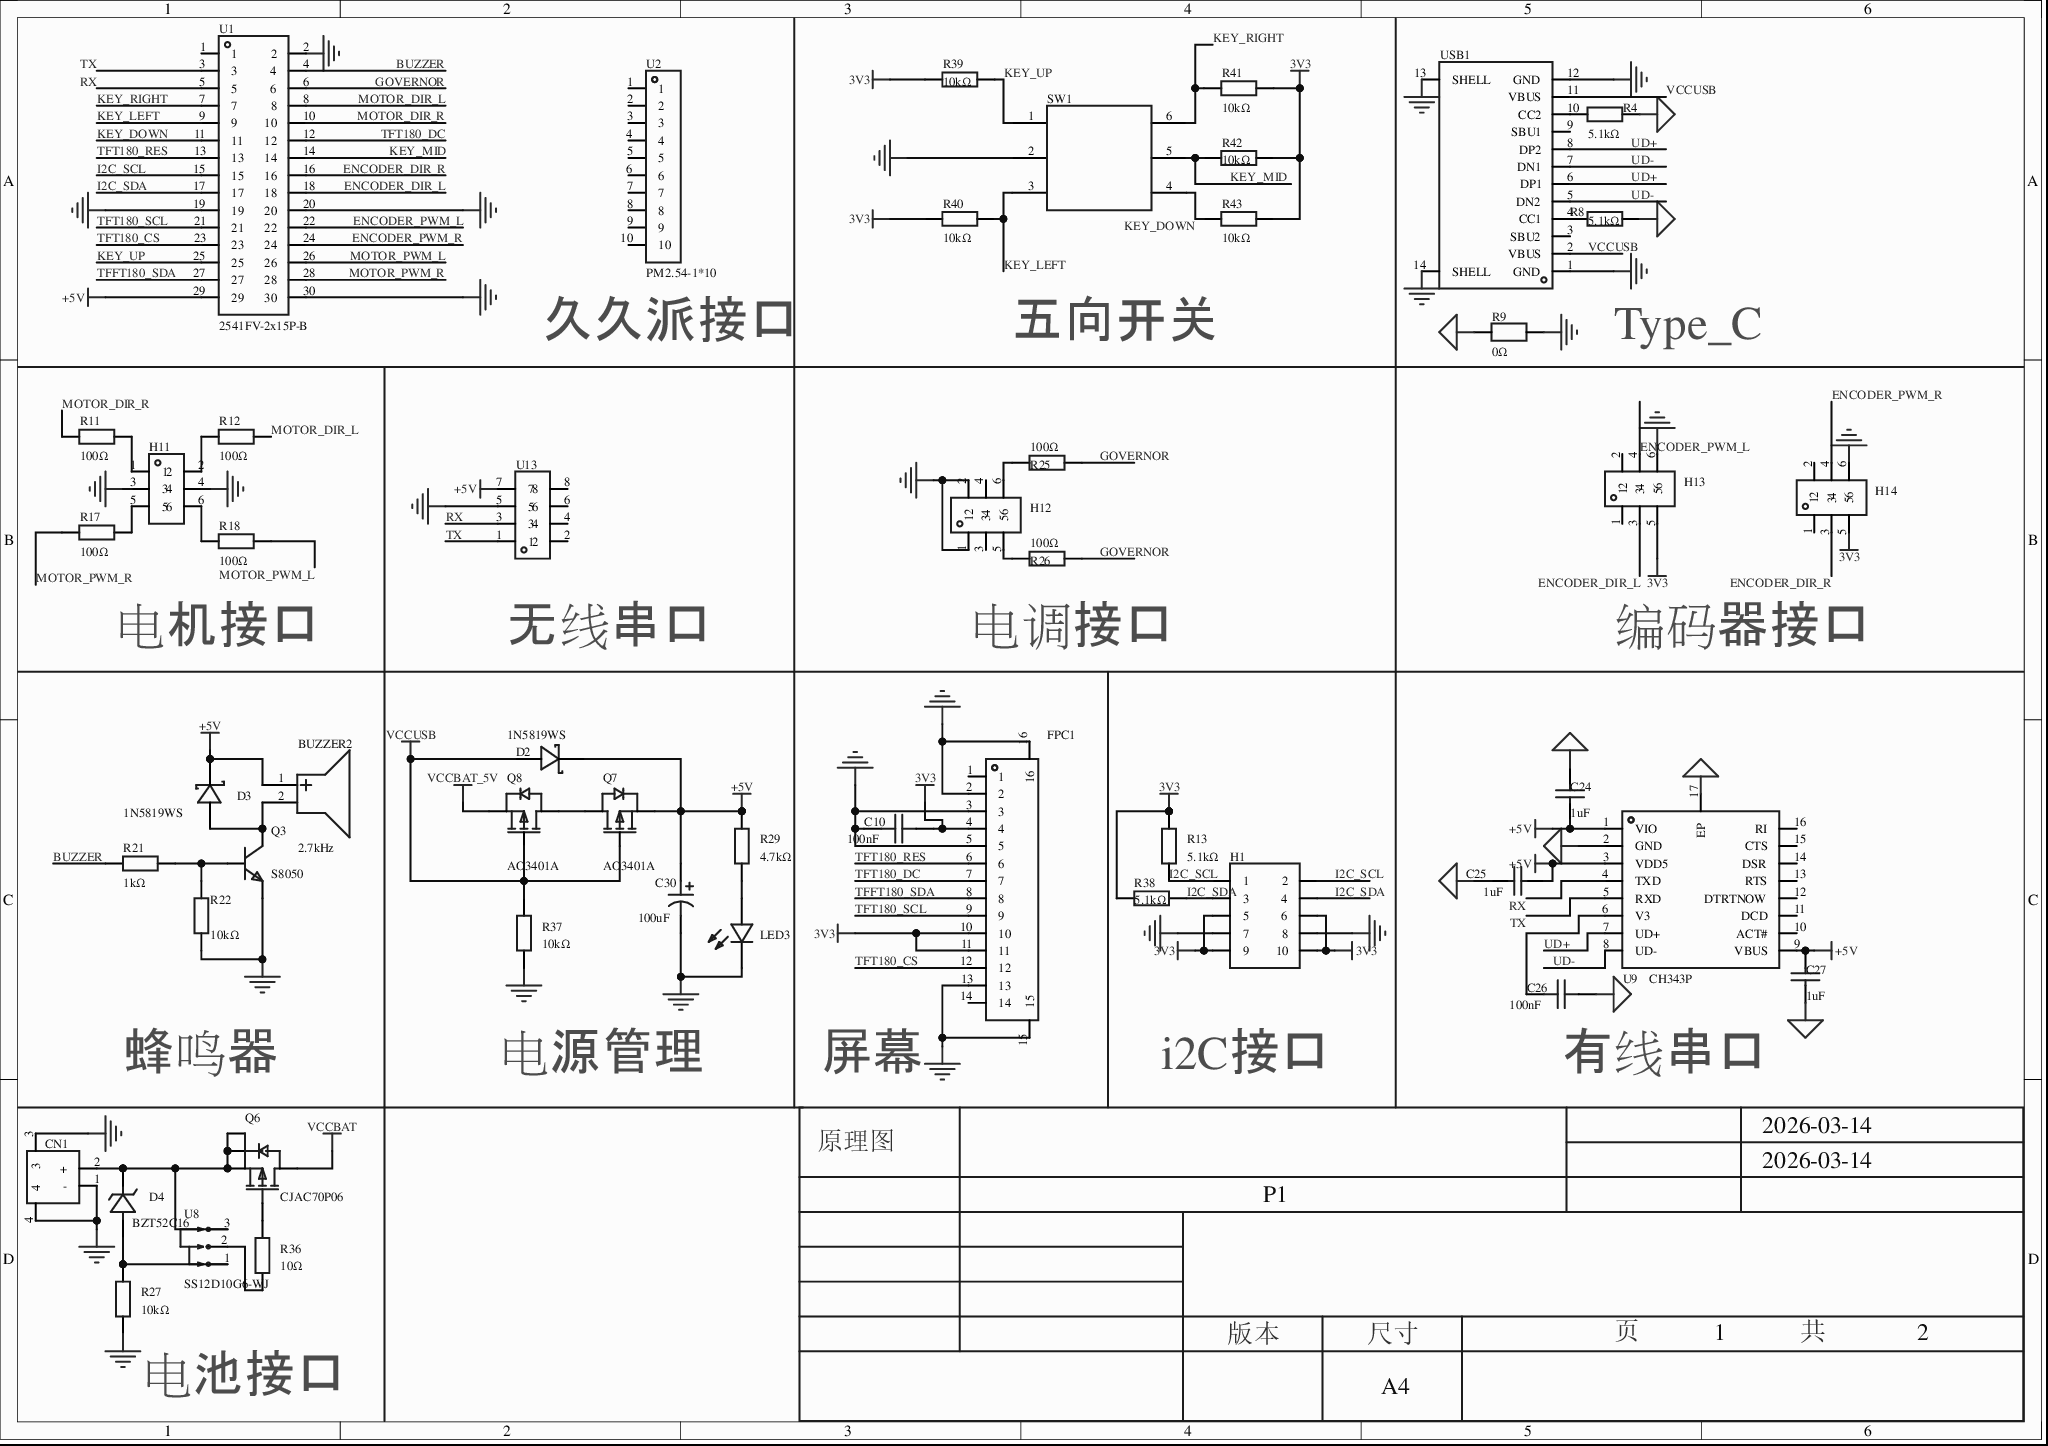
[diagram p0: MISC51977-3.schdoc]
# Altium project MISC51977-2.PrjPcb (part 1 of 2)
2 sheets, 74 parts. Net scope: global (net labels, ports and power ports of the same name join across sheets).
Board file: MISC51977.pcbdoc
Sheets:
  MISC51977-3.schdoc
  MISC51977-4.schdoc

## Sheet MISC51977-3.schdoc
size 297 x 209 mm; Version: V1.0; @Project Name: MISC51977; @Page Count: 2; @Update Date: 2026-03-14; @Create Date: 2026-03-14; @Schematic Name: MISC51977; @Page No: 1; @Board Name: MISC51977; @Create Time: 15:58:27; @Update Time: 22:07:32

### Parts
BUZZER2  2.7kHz  [BUZ-SMD_GSC9032RB]
C10  100nF  [C0603]
C24  1uF  [C0805]
C25  1uF  [C0805]
C26  100nF  [C0603]
C27  1uF  [C0805]
C30  100uF  [CAP-SMD_BD6.3-L6.6-W6.6-FD-1]
CN1  XT30PW-M30.G.Y  [CONN-TH_XT30PW-M]  (value not drawn)
D2  1N5819WS  [SOD-323_L1.8-W1.3-LS2.5-RD]
D3  1N5819WS  [SOD-323_L1.8-W1.3-LS2.5-RD]
D4  BZT52C16  [SOD-123_L2.7-W1.6-LS3.7-RD]
FPC1  HC-FPC-05-09-14RLTAG  [FPC-SMD_14P-P0.50_HC-FPC-05-09-14RLTAG]  (value not drawn)
H1  (no value)  [HDR-TH_10P-P2.54-V-F-R2-C5-S2.54]
H11  HX PZ2.54-2x3P TP  [HDR-SMD_6P-P2.54-V-M-R2-C3-LS7.2_M20-8760342]  (value not drawn)
H12  HX PZ2.54-2x3P TP  [HDR-SMD_6P-P2.54-V-M-R2-C3-LS7.2_M20-8760342]  (value not drawn)
H13  PZ254V-12-6P  [HDR-TH_6P-P2.54-V-M-R2-C3-S2.54]  (value not drawn)
H14  PZ254V-12-6P  [HDR-TH_6P-P2.54-V-M-R2-C3-S2.54]  (value not drawn)
LED3  NCD0603R1  [LED0603-RD_RED]  (value not drawn)
Q3  S8050  [SOT-23-3_L2.9-W1.6-P1.90-LS2.8-BR]
Q6  CJAC70P06  [TDSON-8_L5.9-W5.2-P1.27-BL]
Q7  AO3401A  [SOT-23_L2.9-W1.3-P1.90-LS2.4-BR]
Q8  AO3401A  [SOT-23_L2.9-W1.3-P1.90-LS2.4-BR]
R4  5.1kΩ  [R0603]
R8  5.1kΩ  [R0603]
R9  0Ω  [R1206]
R11  100Ω  [R0603]
R12  100Ω  [R0603]
R13  5.1kΩ  [R0603]
R17  100Ω  [R0603]
R18  100Ω  [R0603]
R21  1kΩ  [R0603]
R22  10kΩ  [R0603]
R25  100Ω  [R0603]
R26  100Ω  [R0603]
R27  10kΩ  [R0603]
R29  4.7kΩ  [R0603]
R36  10Ω  [R0603]
R37  10kΩ  [R0603]
R38  5.1kΩ  [R0603]
R39  10kΩ  [R0603]
R40  10kΩ  [R0603]
R41  10kΩ  [R0603]
R42  10kΩ  [R0603]
R43  10kΩ  [R0603]
SW1  7*7*5-6P-L WX  [SW-SMD_8P-L7.0-W7.0-P1.40-LS7.4-TL]  (value not drawn)
U1  2541FV-2x15P-B  [HDR-TH_30P-P2.54-V-F-R2-C15-S2.54]
U2  PM2.54-1*10  [HDR-TH_10P-P2.54-V-F]
U8  SS12D10G6-WJ  [SW-TH_3P-P4.80_HX-SS12D10G6-WJ]
U9  CH343P  [TQFN-16_L3.0-W3.0-P0.50-BL-EP1.7]
U13  5BME8-08872-204-W0  [CONN-SMD_5BME8-08872-204-W0]  (value not drawn)
USB1  TYPE-C 16PIN 2MD(073)  [USB-C-SMD_TYPE-C-6PIN-2MD-073]  (value not drawn)

### Nets
3V3: C10.2 FPC1.4 FPC1.10 FPC1.11 H1.5 H1.6 H1.9 H1.10 H13.5 H14.5 R13.2 R38.2 R39.1 R40.1 R41.2 R42.2 R43.2
+5V: BUZZER2.1(+) C24.1 C25.1 C27.2 C30.1 D2.1(K) D3.1(K) Q7.2(S) R29.2 U1.29 U9.1(VIO) U9.3(VDD5) U9.9(VBUS) U13.7
AGND: C24.2 C25.2 C26.2 C27.1 R4.2 R8.2 R9.1 U9.2(GND) U9.17(EP)
GND: C10.1 C30.2 CN1.1(-) CN1.3 CN1.4 FPC1.2 FPC1.3 FPC1.5 FPC1.13 FPC1.15 FPC1.16 H1.7 H1.8 H11.3 H11.4 H12.1 H12.2 H13.6 H14.6 LED3.1(K) Q3.2 R9.2 R22.2 R27.1 R37.1 SW1.2 U1.2 U1.19 U1.20 U1.30 U13.5 USB1.1(GND) USB1.12(GND) USB1.13(SHELL) USB1.14(SHELL)
VCCBAT: Q6.5(D)
VCCBAT_5V: Q8.2(S)
VCCUSB: D2.2(A) Q7.1(G) Q8.1(G) R37.2 USB1.2(VBUS) USB1.11(VBUS)
BUZZER: R21.1 U1.4
ENCODER_DIR_L: H13.3 U1.18
ENCODER_DIR_R: H14.3 U1.16
ENCODER_PWM_L: H13.4 U1.22
ENCODER_PWM_R: H14.4 U1.24
GOVERNOR: R25.2 R26.2 U1.6
I2C_SCL: H1.1 H1.2 R13.1 U1.15
I2C_SDA: H1.3 H1.4 R38.1 U1.17
KEY_DOWN: R43.1 SW1.4 U1.11
KEY_LEFT: R40.2 SW1.3 U1.9
KEY_MID: R42.1 SW1.5 U1.14
KEY_RIGHT: R41.1 SW1.6 U1.7
KEY_UP: R39.2 SW1.1 U1.25
MOTOR_DIR_L: R12.2 U1.8
MOTOR_DIR_R: R11.1 U1.10
MOTOR_PWM_L: R18.2 U1.26
MOTOR_PWM_R: R17.1 U1.28
RX: U1.5 U9.4(TXD) U13.3
TFFT180_SDA: FPC1.8 U1.27
TFT180_CS: FPC1.12 U1.23
TFT180_DC: FPC1.7 U1.12
TFT180_RES: FPC1.6 U1.13
TFT180_SCL: FPC1.9 U1.21
TX: U1.3 U9.5(RXD) U13.1
UD+: U9.7(UD+) USB1.6(DP1) USB1.8(DP2)
UD-: U9.8(UD-) USB1.5(DN2) USB1.7(DN1)
NetBUZZER2_2: BUZZER2.2(-) D3.2(A) Q3.3
NetC26_1: C26.1 U9.6(V3)
NetCN1_2: CN1.2(+) D4.1(K) Q6.1(S) Q6.2(S) Q6.3(S) U8.3
NetD4_2: D4.2(A) R27.2 U8.1
NetH11_1: H11.1 R11.2
NetH11_2: H11.2 R12.1
NetH11_5: H11.5 R17.2
NetH11_6: H11.6 R18.1
NetH12_5: H12.5 R26.1
NetH12_6: H12.6 R25.1
NetLED3_2: LED3.2(A) R29.1
NetQ3_1: Q3.1 R21.2 R22.1
NetQ6_4: Q6.4(G) R36.2
NetQ7_3: Q7.3(D) Q8.3(D)
NetR4_1: R4.1 USB1.10(CC2)
NetR8_1: R8.1 USB1.4(CC1)
NetR36_1: R36.1 U8.2

Not connected (* = marked no-connect by the designer): FPC1 1* 14*; H12 3* 4*; H13 1* 2*; H14 1* 2*; U1 1*; U2 1* 2* 3* 4* 5* 6* 7* 8* 9* 10*; U9 10(ACT#)* 11(DCD)* 12(DTRTNOW)* 13(RTS)* 14(DSR)* 15(CTS)* 16(RI)*; U13 2* 4* 6* 8*; USB1 3(SBU2)* 9(SBU1)*

### Notes on the sheet
- (near U2) 久久派接口
- 五向开关
- Type_C
- 电机接口
- (near U13) 无线串口
- 电调接口
- 编码器接口
- 蜂鸣器
- 电源管理
- 屏幕
- i2C接口
- (near C26) 有线串口
- (near R27) 电池接口
- 2026-03-14
- 原理图
- P1
- 版本
- 尺寸
- A4
- 页
- 1
- 共
- 2

### Library data of the parts
BUZZER2 = GSC9032RB-16R2700: 驱动方式:无源(外部驱动);构造类型:电磁式;额定电压:3.6V;频率:2.7kHz;声压(SPL):85dB;; Manufacturer: INGHAi(赢海); AddInBom: yes; ModelId: 6d10ac767011472d9e367b81df9b4b54; ModelName: BUZ-SMD_BD9.0-H3.2-LS10.5; ModelTransform: 413.385,413.385,0,180,0,0,0.002,-29.532,0; Voltage Rating: 3.6V; Voltage - Supply: 2V~4V; Current Consumption: 80mA; Sound Pressure Level(SPL): 85dB; Symbol: GSC9032RB-16R2700; Device: GSC9032RB-16R2700; LCSC Part Name: 贴片式电磁无源蜂鸣器（外部驱动）; SupplierPart: C255321; ManufacturerPart: GSC9032RB-16R2700; Supplier Footprint: -; JLCPCB Part Class: 扩展库; Datasheet: https://item.szlcsc.com/datasheet/GSC9032RB-16R2700/249273.html; Supplier: LCSC; ConvertToPcb: yes; FootprintName: BUZ-SMD_GSC9032RB; Driver Circuitry: 无源(外部驱动); Technology: 电磁式; Value: 2.7kHz; Diameter(φD): 9mm; Height: 3.5mm; Operating Temperature: -20℃~+80℃; Mounting Type: 贴片
C10 C26 = CGA0603X7R104K500JT: 容值:100nF;精度:±10%;额定电压:50V;材质(温度系数):X7R;; Manufacturer: HRE(芯声); AddInBom: yes; ModelId: ac125912035d415993ca9572d50418b1; ModelName: C0603_L1.6-W0.8-H0.8; ModelTransform: 62.992,31.496,0,0,0,0,0,0,0; Tolerance: ±10%; Voltage Rated: 50V; Temperature Coefficient: X7R; Symbol: CGA0603X7R104K500JT; Device: CGA0603X7R104K500JT; LCSC Part Name: 100nF ±10% 50V; SupplierPart: C6119867; ManufacturerPart: CGA0603X7R104K500JT; Supplier Footprint: 0603; JLCPCB Part Class: 扩展库; Supplier: LCSC; ConvertToPcb: yes; FootprintName: C0603; Value: 100nF
C24 C25 C27 = CL21B105KBFNNNE: 容值:1uF;精度:±10%;额定电压:50V;温度系数:X7R;; Manufacturer: SAMSUNG(三星); AddInBom: yes; ModelId: 1ba041120af144c991958decab20d241; ModelName: C0805_L2.0-W1.3-H1.3; ModelTransform: 78.74,51.181,0,0,0,0,0,0.0005,0; Tolerance: ±10%; Voltage Rating: 50V; Temperature Coefficient: X7R; Symbol: CL21B105KBFNNNE; Device: CL21B105KBFNNNE; LCSC Part Name: 1uF ±10% 50V; SupplierPart: C28323; ManufacturerPart: CL21B105KBFNNNE; Supplier Footprint: 0805; JLCPCB Part Class: 基础库; Datasheet: https://item.szlcsc.com/datasheet/CL21B105KBFNNNE/29074.html; Supplier: LCSC; ConvertToPcb: yes; FootprintName: C0805; Value: 1uF
C30 = JVJ25V100M6x5: 容值:100uF;精度:±20%;额定电压:25V;纹波电流:72mA@120Hz;; Manufacturer: JIERR(捷而瑞); AddInBom: yes; ModelId: 041333f082e2432d92aae8a67d233574; ModelTransform: 299.212,259.842,0,0,0,0,0,0,0; Tolerance: ±20%; Voltage Rating: 25V; Lifetime: 2000hrs@105℃; Symbol: JVJ25V100M6X5; Device: JVJ25V100M6x5; LCSC Part Name: 100uF ±20% 25V; SupplierPart: C46550402; ManufacturerPart: JVJ25V100M6x5; Supplier Footprint: SMD,D6.3xL5.4mm; JLCPCB Part Class: 扩展库; Datasheet: https://item.szlcsc.com/datasheet/JVJ25V100M6x5/48680096.html; Supplier: LCSC; ConvertToPcb: yes; FootprintName: CAP-SMD_BD6.3-L6.6-W6.6-FD-1; ModelName: CAP-SMD_BD6.3-L6.6-W6.6-FD-1; Value: 100uF; Ripple Current: 72mA@120Hz; Diameter: 6.3mm; Height - Seated (Max): 5.4mm; Operating Temperature: -55℃~+105℃
CN1 = XT30PW-M30.G.Y: 类别:-;类型1:-;; Manufacturer: AMASS(艾迈斯); AddInBom: yes; ModelId: 722652c2597f41cd937322584dc4b29b; ModelTransform: 523.621,549.2115,0,0,0,0,-0.005,-39.568,-78.74; RatedVoltage: DC 500V; InterfaceType: 公头; RatedCurrent: 15A; RecommendedWireGauge: 16/18/20AWG; contact resistance: 1.2mΩ; specifications: 2pin; Symbol: XT30PW-M; Device: XT30PW-M30.G.Y; LCSC Part Name: AMASS(艾迈斯)航模插头 卧式弯脚 XT30PW-M公头; SupplierPart: C431092; ManufacturerPart: XT30PW-M30.G.Y; Supplier Footprint: -; JLCPCB Part Class: 扩展库; Datasheet: https://atta.szlcsc.com/upload/public/pdf/source/20220222/6A9F22F7850E25B33E1BE430ADF8560B.pdf; Supplier: LCSC; ConvertToPcb: yes; FootprintName: CONN-TH_XT30PW-M; ModelName: CONN-TH_XT30PW-M; Power: -; Output: -; Input: -; Size: -; Interface: -; Type: 航模插头; Colour: -; MaximumCurrent: -; Type1: -; NumberOfUSBHoles: -; MetalMaterial: -; InsulationMaterial: -; FlameRetardantGrade: -; Belt length: -
D2 D3 = 1N5819WS_C191023: 正向压降(Vf):600mV@1A;直流反向耐压(Vr):40V;整流电流:1A;; Manufacturer: Hottech(合科泰); AddInBom: yes; ModelId: 7459fe65e23146c0a8d836e46a0add72; ModelTransform: 104.3305,51.181,0,0,0,0,0,0,0; Voltage - DC Reverse(Vr): 40V; Current - Rectified: 1A; Non-Repetitive Peak Forward Surge Current: 25A; Symbol: 1N5819WS; Device: 1N5819WS_C191023; LCSC Part Name: 电压:40V 电流:1A; SupplierPart: C191023; ManufacturerPart: 1N5819WS; Supplier Footprint: SOD-323; JLCPCB Part Class: 基础库; Datasheet: https://item.szlcsc.com/datasheet/1N5819WS/213850.html; Supplier: LCSC; ConvertToPcb: yes; FootprintName: SOD-323_L1.8-W1.3-LS2.5-RD; ModelName: SOD-323_L1.8-W1.3-LS2.5-RD; Voltage - Forward(Vf@If): 600mV@1A
D4 = BZT52C16_C19077413: 二极管配置:独立式;稳压值(标称值):16V;稳压值(范围):15.2V~16.8V;耗散功率(Pd):500mW;; Manufacturer: 宏嘉诚; AddInBom: yes; ModelId: ad7e39f9e5534b3c96ffdc5532ebb493; ModelName: SOD-123_L2.7-W1.6-H1.4-LS3.7; ModelTransform: 146.026,62.992,0,180,0,0,0.0005,0,0; Diode Configuration: 独立式; Zener Voltage(Nom): 16V; Reverse Leakage Current (Ir): 100nA@11.2V; Pd - Power Dissipation(Pd): 500mW; Impedance(Zzt): 45Ω; Symbol: BZT52C16_C19077413; Device: BZT52C16_C19077413; LCSC Part Name: BZT52C16; SupplierPart: C19077413; ManufacturerPart: BZT52C16; Supplier Footprint: SOD-123; JLCPCB Part Class: 扩展库; Datasheet: https://atta.szlcsc.com/upload/public/pdf/source/20250106/E12AA82D484C9C66E469D005F460C1F7.pdf; Supplier: LCSC; ConvertToPcb: yes; FootprintName: SOD-123_L2.7-W1.6-LS3.7-RD; Zener Voltage(Range): 15.2V~16.8V
FPC1 = HC-FPC-05-09-14RLTAG: 锁定特性:翻盖式;触点类型:双侧触点/上下接;触点数量:14P;间距:0.5mm;安装方式:卧贴;工作温度:-55℃~+85℃;; Manufacturer: HCTL(华灿天禄); AddInBom: yes; ModelId: 24765ce4246b49c98a108f81db7afb13; ModelTransform: 354.7237,137.795,0,180,0,0,0,-1.732,0; Locking Feature: 翻盖式; Number of Contacts: 14P; Pitch: 0.5mm; FFC, FCB Thickness: 0.3mm; Symbol: HC-FPC-05-09-14RLTAG; Device: HC-FPC-05-09-14RLTAG; LCSC Part Name: 翻盖式 双侧触点/上下接 P数:14P 间距:0.5mm; SupplierPart: C5213752; ManufacturerPart: HC-FPC-05-09-14RLTAG; Supplier Footprint: SMD,P=0.5mm,卧贴; JLCPCB Part Class: 扩展库; Datasheet: https://item.szlcsc.com/datasheet/HC-FPC-05-09-14RLTAG/5909044.html; Supplier: LCSC; ConvertToPcb: yes; FootprintName: FPC-SMD_14P-P0.50_HC-FPC-05-09-14RLTAG; ModelName: FPC-SMD_14P-P0.50_HC-FPC-05-09-14RLTAG; Contact Type: 双侧触点/上下接; Mounting Type: 卧贴; Height Above Board: 1mm; Contact Material: 铜合金; Operating Temperature: -55℃~+85℃
H1 = HDR-F_2.54_2x5: Symbol: HDR-F-2.54_2x5; ConvertToPcb: yes; ModelId: 86e5d65f54dd476391caab3fdb9168240819f05c4eef4c71ace90d822a990e87; ModelName: HDR2.54-F-LI-2X5P; ModelTransform: 499.999,200,0,0,0,0,0,0,-118.11; Device: HDR-F_2.54_2x5; AddInBom: yes; SupplierPart: C92270; Supplier Footprint: 插件; FootprintName: HDR-TH_10P-P2.54-V-F-R2-C5-S2.54
H11 H12 = HX PZ2.54-2x3P TP: 插针结构:2x3P;间距:2.54mm;行距:2.54mm;圆针/方针:方针;安装方式:立贴;排数:双排;总PIN位数:6P;额定电流:3A;额定电压:1kV;配合针长度:6mm;塑高:2.5mm;端接针长度:-;触头材质:黄铜;触头镀层:金;工作温度:-40℃~+105℃;颜色:黑色;; Manufacturer: hanxia(韩下); AddInBom: yes; ModelId: e8488307e3c0448d924ff5d10fcc2db3; ModelTransform: 299.9994,283.464,0,0,0,0,0,0,0; Pin Structure: 2x3P; Pitch: 2.54mm; Circluar Pins/Square Pins: 方针; Current Rating: 3A; Voltage Rating (Max): 1kV; Symbol: HX PZ2.54-2X3P TP; Device: HX PZ2.54-2x3P TP; LCSC Part Name: 2x3P 间距:2.54mm 方针 立贴; SupplierPart: C32713283; ManufacturerPart: HX PZ2.54-2x3P TP; Supplier Footprint: SMD,P=2.54mm; JLCPCB Part Class: 扩展库; Datasheet: https://item.szlcsc.com/datasheet/HX%2520PZ2.54-2x3P%2520TP/34444563.html; Supplier: LCSC; ConvertToPcb: yes; FootprintName: HDR-SMD_6P-P2.54-V-M-R2-C3-LS7.2_M20-8760342; ModelName: HDR-SMD_6P-P2.54-V-M-R2-C3-LS7.2_M20-8760342; Row Spacing: 2.54mm; Mounting Type: 立贴; Number of Rows: 双排; Number of Pins: 6P; Length of Mating Pin: 6mm; Insulation Height: 2.5mm; Length of End Connection Pin: -; Contact Material: 黄铜; Contact Plating: 金; Operating Temperature: -40℃~+105℃; Color: 黑色; Supplementary Features: -
H13 H14 = PZ254V-12-6P: 插针结构:2x3P;间距:2.54mm;行距:2.54mm;圆针/方针:方针;安装类型:直插;排数:双排;总PIN位数:6P;额定电流:-;额定电压:-;配合针长度:6mm;塑高:2.5mm;端接针长度:3mm;触头材质:黄铜;触头镀层:-;工作温度范围:-40℃~+105℃;颜色:黑色;; Manufacturer: XFCN(兴飞); AddInBom: yes; ModelId: e22692306cbd4b5c8488f4142eed6b9c; ModelTransform: 300.3931,200,0,0,0,0,0,0,-118.11; Pin Structure: 2x3P; Pitch: 2.54mm; Circluar Pins/Square Pins: 方针; Symbol: PZ254V-12-6P; Device: PZ254V-12-6P; LCSC Part Name: 间距:2.54mm 2x3P 直插 方针; SupplierPart: C492420; ManufacturerPart: PZ254V-12-6P; Supplier Footprint: 插件,P=2.54mm; JLCPCB Part Class: 扩展库; Datasheet: https://atta.szlcsc.com/upload/public/pdf/source/20200309/C492420_BAECB307B001054C09D200388220EAE6.pdf; Supplier: LCSC; ConvertToPcb: yes; FootprintName: HDR-TH_6P-P2.54-V-M-R2-C3-S2.54; ModelName: HDR-TH_6P-P2.54-V-M-R2-C3-S2.54; Row Spacing: 2.54mm; Mounting Type: 直插; Number of Rows: 双排; Number of Pins: 6P; Current Rating (Max): -; Voltage Rating (Max): -; Length of Mating Pin: 6mm; Insulation Height: 2.5mm; Length of End Connection Pin: 3mm; Contact Material: 黄铜; Contact Plating: -; Operating Temperature Range: -40℃~+105℃; Color: 黑色
LED3 = NCD0603R1_C84263: 灯头类型:-;发光颜色:红色;正向电压(VF):1.6V~2.6V;功率:65mW;正向电流:20mA;主波长:615nm~630nm;二极管配置:独立二极管;透镜颜色:无色透明透镜;色温:-;发光强度:80mcd~220mcd;发光角度:130°;载带方式:-;工作温度:-30℃~+85℃;; Manufacturer: 国星光电; Symbol: FC-DA1608HRK-620D; AddInBom: yes; ModelId: 74041d3a270d435c8600a9ab9b7641c0; ModelTransform: 63.7794,31.496,0,0,0,0,0,0,0; Emitted Color: 红色; Power Dissipation: 65mW; Forward Current: 20mA; Diode Configuration: 独立二极管; Lens Color: 无色透明透镜; Viewing Angle: 130°; Device: NCD0603R1_C84263; LCSC Part Name: NCD0603R1; SupplierPart: C84263; ManufacturerPart: NCD0603R1; Supplier Footprint: 0603; JLCPCB Part Class: 扩展库; Datasheet: https://atta.szlcsc.com/upload/public/pdf/source/20200820/C84263_DABC6A75E58F576973B407FDBA283D60.pdf; Supplier: LCSC; ConvertToPcb: yes; FootprintName: LED0603-RD_RED; ModelName: LED0603-RD_RED; Lamp Holder Type: -; Forward Voltage (VF): 1.6V~2.6V; Dominant Wavelength: 615nm~630nm; Peak Wavelength: -; Color Temperature: -; Luminous Intensity: 80mcd~220mcd; Mounting Sytle: -; Operating Temperature: -30℃~+85℃
Q3 = S8050_C181158: 晶体管类型:NPN;集电极电流(Ic):500mA;集射极击穿电压(Vceo):25V;功率(Pd):300mW;; Manufacturer: Hottech(合科泰); AddInBom: yes; ModelId: 89cb27a44ab2466697082bb9fd73a7d0; ModelName: SOT-23-3L_L2.9-W1.6-H1.1-LS2.8-P0.95; ModelTransform: 114.173,110.236,0,90,0,0,0,0,0; Transistor Type: NPN; Collector Current (Ic): 500mA; Collector-Emitter Breakdown Voltage (Vceo): 25V; Power Dissipation (Pd): 300mW; Transition Frequency (fT): 150MHz; Collector Cut-Off Current (Icbo): 100nA; Collector-Emitter Saturation Voltage (VCE(sat)@Ic,Ib): 600mV@500mA,50mA; Symbol: S8050_C181158; Device: S8050_C181158; LCSC Part Name: NPN 电流:500mA 耐压:25V H档; SupplierPart: C181158; ManufacturerPart: S8050; Supplier Footprint: SOT-23; JLCPCB Part Class: 扩展库; Datasheet: https://atta.szlcsc.com/upload/public/pdf/source/20220506/D987F39D56F2975D34EC7947E75C4ABC.pdf; Supplier: LCSC; ConvertToPcb: yes; FootprintName: SOT-23-3_L2.9-W1.6-P1.90-LS2.8-BR; Operating Temperature: -
Q6 = CJAC70P06: 类型:1个P沟道;漏源电压(Vdss):60V;连续漏极电流(Id):70A;导通电阻(RDS(on)@Vgs,Id):9.2mΩ@4.5V,10A;功率(Pd):115W;阈值电压(Vgs(th)@Id):1V@250uA;; Manufacturer: CJ(江苏长电/长晶); AddInBom: yes; ModelId: ff3d8edf19694f3eb1c5df98919f3bc8; ModelTransform: 216.9287,242.5192,0,0,0,0,0,43.307,0; Type: 1个P沟道; Drain Source Voltage (Vdss): 60V; Continuous Drain Current (Id): 70A; Power Dissipation (Pd): 115W; Total Gate Charge (Qg@Vgs): 210nC@10V; Input Capacitance (Ciss@Vds): 12.5nF@30V; Reverse Transfer Capacitance (Crss@Vds): 430pF@30V; Symbol: CJAC70P06; Device: CJAC70P06; LCSC Part Name: 1个P沟道 耐压:60V 电流:70A; SupplierPart: C2898279; ManufacturerPart: CJAC70P06; Supplier Footprint: PDFNWB-8L-EP(5x6); JLCPCB Part Class: 扩展库; Datasheet: https://atta.szlcsc.com/upload/public/pdf/source/20210915/A7D9F10F1676D48BCD8F5D63B1C65749.pdf; Supplier: LCSC; ConvertToPcb: yes; FootprintName: TDSON-8_L5.9-W5.2-P1.27-BL; ModelName: TDSON-8_L5.9-W5.2-P1.27-BL; Drain Source On Resistance (RDS(on)@Vgs,Id): 9.2mΩ@4.5V,10A; Gate Threshold Voltage (Vgs(th)@Id): 1V@250uA; Operating Temperature: -55℃~+150℃
Q7 Q8 = AO3401A_C347476: 数量:1个P沟道;漏源电压(Vdss):30V;连续漏极电流(Id):4.2A;导通电阻(RDS(on)):50mΩ@10V;耗散功率(Pd):1.4W;阈值电压(Vgs(th)):1.3V@250uA;; Manufacturer: UMW(友台半导体); AddInBom: yes; ModelId: c62791f0466c4ae2a892c056b845b0ca; ModelName: SOT-23-3P_L2.9-W1.3-H1.0-LS2.4-P0.95; ModelTransform: 98.64468,114.173,0,180,0,0,0,0,0; Number: 1个P沟道; Drain to Source Voltage: 30V; Current - Continuous Drain(Id): 4.2A; Pd - Power Dissipation: 1.4W; Gate Charge(Qg): 9.4nC@4.5V; Input Capacitance(Ciss): 954pF; Reverse Transfer Capacitance (Crss@Vds): 77pF; Type: P沟道; Output Capacitance(Coss): 115pF; Symbol: AO3401A_C347476; Device: AO3401A_C347476; LCSC Part Name: 1个P沟道 耐压:30V 电流:4.2A; SupplierPart: C347476; ManufacturerPart: AO3401A; Supplier Footprint: SOT-23; JLCPCB Part Class: 扩展库; Datasheet: https://item.szlcsc.com/datasheet/AO3401A/324136.html; Supplier: LCSC; ConvertToPcb: yes; FootprintName: SOT-23_L2.9-W1.3-P1.90-LS2.4-BR; RDS(on): 50mΩ@10V; Gate Threshold Voltage (Vgs(th)): 1.3V@250uA; Operating Temperature: -55℃~+150℃
R4 R8 R13 R38 = 0603WAF5101T5E: 电阻类型:厚膜电阻;阻值:5.1kΩ;精度:±1%;功率:100mW;最大工作电压:75V;温度系数:±100ppm/℃;; Manufacturer: UNI-ROYAL(厚声); AddInBom: yes; ModelId: fc143cca1e79419f9cd78b61e9279f08; ModelTransform: 31.8897,63.7794,0,90,0,0,0,0,0; Tolerance: ±1%; Power(Watts): 100mW; Overload Voltage (Max): 75V; Symbol: 0603WAF5101T5E; Device: 0603WAF5101T5E; LCSC Part Name: 5.1kΩ ±1% 100mW 厚膜电阻; SupplierPart: C23186; ManufacturerPart: 0603WAF5101T5E; Supplier Footprint: 0603; JLCPCB Part Class: 基础库; Datasheet: https://atta.szlcsc.com/upload/public/pdf/source/20200306/C422600_1E6D84923E4A46A82E41ADD87F860B5C.pdf; Supplier: LCSC; ConvertToPcb: yes; FootprintName: R0603; ModelName: R0603; Type: 厚膜电阻; Value: 5.1kΩ; Temperature Coefficient: ±100ppm/℃; Operating Temperature Range: -55℃~+155℃
R9 = FRC1206P000 TS: 电阻类型:厚膜电阻;阻值:0Ω;精度:±5%;功率:250mW;最大工作电压:200V;; Manufacturer: FOJAN(富捷); AddInBom: yes; ModelId: 89a1f13db2384da588040e0b3c55bf66; ModelName: R1206_L3.2-W1.6-H0.6; ModelTransform: 125.984,62.992,0,0,0,0,0,0,0; Tolerance: ±5%; Power(Watts): 250mW; Overload Voltage (Max): 200V; Symbol: FRC1206P000 TS; Device: FRC1206P000 TS; LCSC Part Name: 0Ω ±5% 250mW 厚膜电阻; SupplierPart: C2907406; ManufacturerPart: FRC1206P000 TS; Supplier Footprint: 1206; JLCPCB Part Class: 扩展库; Datasheet: https://atta.szlcsc.com/upload/public/pdf/source/20211221/925EC7D7225764EE0046F22065062C87.pdf; Supplier: LCSC; ConvertToPcb: yes; FootprintName: R1206; Type: 厚膜电阻; Value: 0Ω; Operating Temperature Range: -55℃~+155℃
R11 R12 R17 R18 R25 R26 = 0603WAF1000T5E: 电阻类型:厚膜电阻;阻值:100Ω;精度:±1%;功率:100mW;最大工作电压:75V;温度系数:±200ppm/℃;; Manufacturer: UNI-ROYAL(厚声); AddInBom: yes; ModelId: fc143cca1e79419f9cd78b61e9279f08; ModelTransform: 31.8897,63.7794,0,90,0,0,0,0,0; Tolerance: ±1%; Power(Watts): 100mW; Overload Voltage (Max): 75V; Symbol: 0603WAF1000T5E; Device: 0603WAF1000T5E; LCSC Part Name: 100Ω ±1% 100mW 厚膜电阻; SupplierPart: C22775; ManufacturerPart: 0603WAF1000T5E; Supplier Footprint: 0603; JLCPCB Part Class: 基础库; Datasheet: https://atta.szlcsc.com/upload/public/pdf/source/20200306/C422600_1E6D84923E4A46A82E41ADD87F860B5C.pdf; Supplier: LCSC; ConvertToPcb: yes; FootprintName: R0603; ModelName: R0603; Type: 厚膜电阻; Value: 100Ω; Temperature Coefficient: ±200ppm/℃; Operating Temperature Range: -55℃~+155℃
R21 = 0603WAF1001T5E: 电阻类型:厚膜电阻;阻值:1kΩ;精度:±1%;功率:100mW;工作电压:75V;温度系数:±100ppm/℃;; Manufacturer: UNI-ROYAL(厚声); AddInBom: yes; ModelId: fc143cca1e79419f9cd78b61e9279f08; ModelTransform: 31.8897,63.7794,0,90,0,0,0,0,0; Tolerance: ±1%; Power(Watts): 100mW; Voltage-Supply(Max): 75V; Symbol: 0603WAF1001T5E; Device: 0603WAF1001T5E; LCSC Part Name: 1kΩ ±1% 100mW 厚膜电阻; SupplierPart: C21190; ManufacturerPart: 0603WAF1001T5E; Supplier Footprint: 0603; JLCPCB Part Class: 基础库; Datasheet: https://item.szlcsc.com/datasheet/0603WAF1001T5E/21904.html; Supplier: LCSC; ConvertToPcb: yes; FootprintName: R0603; ModelName: R0603; Type: 厚膜电阻; Value: 1kΩ; Temperature Coefficient: ±100ppm/℃; Operating Temperature: -55℃~+155℃
R22 R27 R37 R39-R43 = 0603WAF1002T5E: 电阻类型:厚膜电阻;阻值:10kΩ;精度:±1%;功率:100mW;最大工作电压:75V;温度系数:±100ppm/℃;; Manufacturer: UNI-ROYAL(厚声); AddInBom: yes; ModelId: fc143cca1e79419f9cd78b61e9279f08; ModelTransform: 31.8897,63.7794,0,90,0,0,0,0,0; Tolerance: ±1%; Power(Watts): 100mW; Overload Voltage (Max): 75V; Symbol: 0603WAF1002T5E; Device: 0603WAF1002T5E; LCSC Part Name: 厚膜电阻 10kΩ ±1% 100mW; SupplierPart: C25804; ManufacturerPart: 0603WAF1002T5E; Supplier Footprint: 0603; JLCPCB Part Class: 基础库; Datasheet: https://atta.szlcsc.com/upload/public/pdf/source/20200306/C422600_1E6D84923E4A46A82E41ADD87F860B5C.pdf; Supplier: LCSC; ConvertToPcb: yes; FootprintName: R0603; ModelName: R0603; Type: 厚膜电阻; Value: 10kΩ; Temperature Coefficient: ±100ppm/℃; Operating Temperature Range: -55℃~+155℃
R29 = 0603WAF4701T5E: 电阻类型:厚膜电阻;阻值:4.7kΩ;精度:±1%;功率:100mW;最大工作电压:75V;温度系数:±100ppm/℃;; Manufacturer: UNI-ROYAL(厚声); AddInBom: yes; ModelId: fc143cca1e79419f9cd78b61e9279f08; ModelTransform: 31.8897,63.7794,0,90,0,0,0,0,0; Tolerance: ±1%; Power(Watts): 100mW; Overload Voltage (Max): 75V; Symbol: 0603WAF4701T5E; Device: 0603WAF4701T5E; LCSC Part Name: 4.7kΩ ±1% 100mW 厚膜电阻; SupplierPart: C23162; ManufacturerPart: 0603WAF4701T5E; Supplier Footprint: 0603; JLCPCB Part Class: 基础库; Datasheet: https://atta.szlcsc.com/upload/public/pdf/source/20200306/C422600_1E6D84923E4A46A82E41ADD87F860B5C.pdf; Supplier: LCSC; ConvertToPcb: yes; FootprintName: R0603; ModelName: R0603; Type: 厚膜电阻; Value: 4.7kΩ; Temperature Coefficient: ±100ppm/℃; Operating Temperature Range: -55℃~+155℃